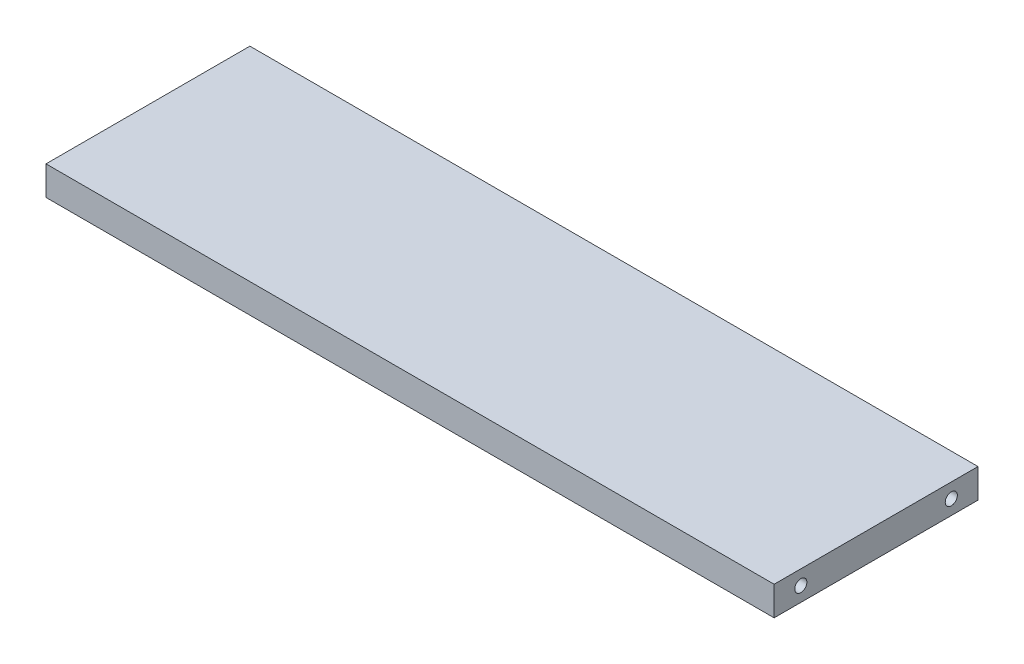
from build123d import *

# Parameters (mm, degrees)
SKETCH1_W             = 150
SKETCH1_H             = 42
BOSS_EXTRUDE1_DEPTH   = 6
SKETCH2_R             = 1.25
CUT_EXTRUDE1_DEPTH    = 5
CUT_EXTRUDE2_START    = -5
SKETCH3_R             = 1.25
CUT_EXTRUDE2_DEPTH    = 5
M3_TAPPED_HOLE1_D     = 2.5
M3_TAPPED_HOLE1_DEPTH = 7.5
M3_TAPPED_HOLE1_TIP   = 0.751075774
M3_TAPPED_HOLE2_D     = 2.5
M3_TAPPED_HOLE2_DEPTH = 7.5
M3_TAPPED_HOLE2_TIP   = 0.751075774


with BuildPart() as part:
    # Sketch1 → Boss-Extrude1 (new body)
    with BuildSketch(Plane(origin=(0, 0, 0), x_dir=(1, 0, 0), z_dir=(0, 1, 0))):
        Rectangle(SKETCH1_W, SKETCH1_H)
    extrude(amount=BOSS_EXTRUDE1_DEPTH)

    # Sketch2 → Cut-Extrude1 (cut)
    with BuildSketch(Plane(origin=(75, 0, 0), x_dir=(0, 0, -1), z_dir=(1, 0, 0))):
        with Locations((15.5, 3)):
            Circle(SKETCH2_R)
        with Locations((-15.5, 3)):
            Circle(SKETCH2_R)
    extrude(amount=-CUT_EXTRUDE1_DEPTH, mode=Mode.SUBTRACT)

    # Sketch3 → Cut-Extrude2 (cut)
    with BuildSketch(Plane.ZY.offset(75).offset(CUT_EXTRUDE2_START)):
        with Locations(Location((-15.5, 3, 0), (0, 0, 180))):
            Circle(SKETCH3_R)
        with Locations(Location((15.5, 3, 0), (0, 0, 180))):
            Circle(SKETCH3_R)
    extrude(amount=CUT_EXTRUDE2_DEPTH, mode=Mode.SUBTRACT)

    # M3 Tapped Hole1
    with Locations(Plane(origin=(75, 0, 0), x_dir=(0, 0, -1), z_dir=(1, 0, 0))):
        with Locations((-15.5, 3), (15.5, 3)):
            Hole(M3_TAPPED_HOLE1_D / 2, depth=M3_TAPPED_HOLE1_DEPTH)
            with Locations((0, 0, -(M3_TAPPED_HOLE1_DEPTH + M3_TAPPED_HOLE1_TIP / 2))):  # 118° drill point
                Cone(0, M3_TAPPED_HOLE1_D / 2, M3_TAPPED_HOLE1_TIP, mode=Mode.SUBTRACT)

    # M3 Tapped Hole2
    with Locations(Plane.ZY.offset(75)):
        with Locations((-15.5, 3), (15.5, 3)):
            Hole(M3_TAPPED_HOLE2_D / 2, depth=M3_TAPPED_HOLE2_DEPTH)
            with Locations((0, 0, -(M3_TAPPED_HOLE2_DEPTH + M3_TAPPED_HOLE2_TIP / 2))):  # 118° drill point
                Cone(0, M3_TAPPED_HOLE2_D / 2, M3_TAPPED_HOLE2_TIP, mode=Mode.SUBTRACT)


solid = part.part
